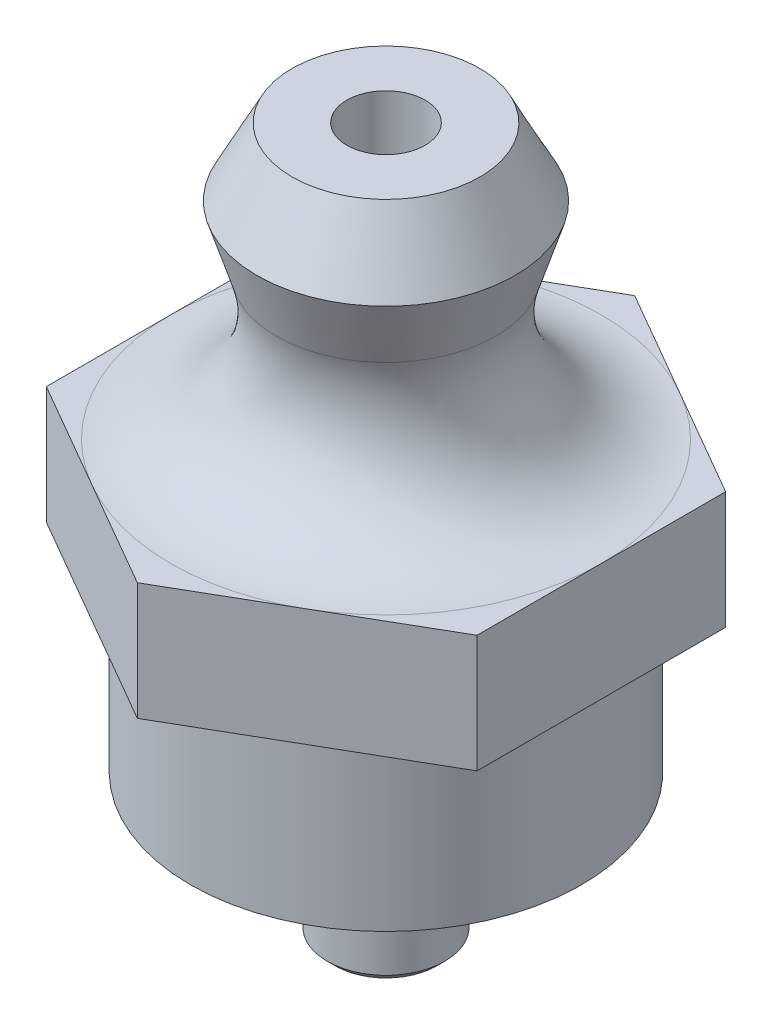
from build123d import *

# Parameters (mm, degrees)
EXTRUDE_1_DEPTH = 3
CHAMFER_1_SIZE  = 0.2


with BuildPart() as part:
    # 草图1 → 旋转2 (revolve)
    with BuildSketch(Plane.XY, mode=Mode.PRIVATE) as revolve_2_sk:
        with BuildLine():
            Line((-1, 18), (-2.4, 18))
            Line((-2.4, 18), (-3.3, 16.271116086))
            Line((-3.3, 16.271116086), (-2.8, 14.675583457))
            ThreePointArc((-2.8, 14.675583457), (-3.219653878, 12.154380629), (-5.5, 11))
            Line((-5.5, 11), (-5.5, 8))
            Line((-5.5, 8), (-5, 8))
            Line((-5, 8), (-5, 3.643969354))
            Line((-5, 3.643969354), (-1.5, 1.821984677))
            Line((-1.5, 1.821984677), (-1.5, 0))
            Line((-1.5, 0), (-1, 0))
            Line((-1, 0), (-1, 18))
        make_face()
    revolve(revolve_2_sk.sketch.rotate(Axis((0, 0, 0), (0, -1, 0)), 270), axis=Axis((0, 0, 0), (0, -1, 0)))

    # 草图2 → 拉伸1 (add)
    with BuildSketch(Plane.XZ.offset(-8)):
        Polygon((-5.5, 3.175426481), (-5.5, -3.175426481), (0, -6.350852961), (5.5, -3.175426481), (5.5, 3.175426481), (0, 6.350852961), align=None)
    extrude(amount=-EXTRUDE_1_DEPTH)

    # 倒角1
    chamfer_1_edges = [part.edges().sort_by_distance(p)[0] for p in [
        (0, 0, -1.5),
    ]]
    chamfer(chamfer_1_edges, length=CHAMFER_1_SIZE)


solid = part.part
